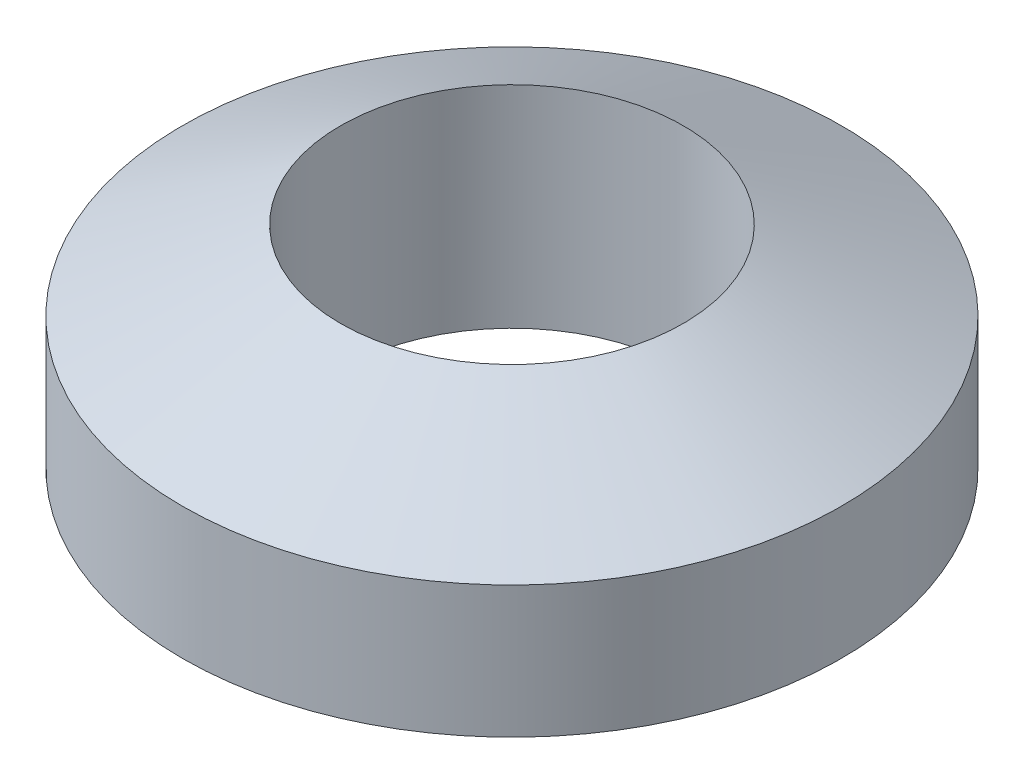
SolidWorks part; units mm, degrees
ref_plane "前视基准面" through (0, 0, 0) normal (0, 0, 1) x (1, 0, 0)
ref_plane "上视基准面" through (0, 0, 0) normal (0, 1, 0) x (1, 0, 0)
ref_plane "右视基准面" through (0, 0, 0) normal (1, 0, 0) x (0, 0, -1)
sketch "草图1" plane through (0, 0, 0) normal (0, 0, 1) x (1, 0, 0)
  line L0 (0, 116.8952) -> (0, -128.4274) construction
  line L1 (65, -53.9919) -> (65, 26.0081)
  line L2 (65, 26.0081) -> (125, -3.9919)
  line L3 (125, -3.9919) -> (125, -53.9919)
  line L4 (125, -53.9919) -> (65, -53.9919)
  dimension "D1" = 65
  dimension "D2" = 60
  dimension "D3" = 50
  dimension "D4" = 80
revolve "旋转1" add sketch "草图1" angle 360 about L0
sketch "草图2" plane through (0, -53.9919, 0) normal (0, -1, 0) x (1, 0, 0)
  circle A0 centre (90, 0) radius 5
  circle A1 centre (63.6396, -63.6396) radius 5
  circle A2 centre (0, -90) radius 5
  circle A3 centre (-63.6396, -63.6396) radius 5
  circle A4 centre (-90, 0) radius 5
  circle A5 centre (-63.6396, 63.6396) radius 5
  circle A6 centre (0, 90) radius 5
  circle A7 centre (63.6396, 63.6396) radius 5
  point P19 (0, 0)
  dimension "D1" = 10
  dimension "D2" = 90
  dimension "D3" = 8
extrude "切除-拉伸1" cut sketch "草图2" against normal blind 30
